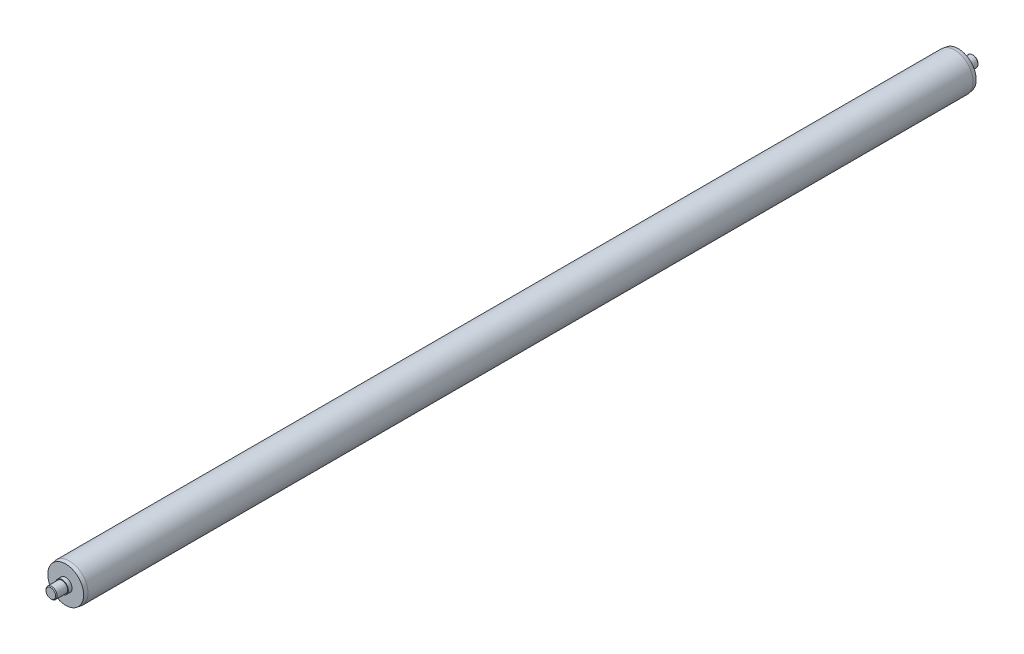
from build123d import *

# Parameters (mm, degrees)
CHAMFER1_SIZE  = 5
CHAMFER1_SIZE2 = 0.881634904
CHAMFER2_SIZE  = 1
SKETCH5_W      = 15.5
SKETCH5_H      = 1184


with BuildPart() as part:
    # Sketch3 → Revolve1 (revolve)
    with BuildSketch(Plane(origin=(0, 0, 0), x_dir=(0, 0, -1), z_dir=(1, 0, 0)), mode=Mode.PRIVATE) as revolve1_sk:
        Polygon((-300, 25), (900, 25), (900, 8.5), (905, 8.5), (905, 7.5), (920, 7.5), (920, 0), (-320, 0), (-320, 7.5), (-305, 7.5), (-305, 8.5), (-300, 8.5), align=None)
    revolve(revolve1_sk.sketch.rotate(Axis((0, 0, 320), (0, 0, -1)), 90), axis=Axis((0, 0, 320), (0, 0, -1)))

    # Chamfer1
    chamfer1_edges = [part.edges().sort_by_distance(p)[0] for p in [
        (-25, 0, -900),
        (-25, 0, 300),
    ]]
    chamfer1_side = [part.faces().sort_by_distance(p)[0] for p in [
        (-25, 0, -300),
    ]]
    chamfer(chamfer1_edges, length=CHAMFER1_SIZE, length2=CHAMFER1_SIZE2, reference=chamfer1_side[0])

    # Chamfer2
    chamfer2_edges = [part.edges().sort_by_distance(p)[0] for p in [
        (-7.5, 0, -920),
        (-7.5, 0, 320),
    ]]
    chamfer(chamfer2_edges, length=CHAMFER2_SIZE)

    # Sketch5 → Cut-Revolve1 (revolve, cut)
    with BuildSketch(Plane(origin=(0, 0, 0), x_dir=(1, 0, 0), z_dir=(0, 1, 0)), mode=Mode.PRIVATE) as cut_revolve1_sk:
        with Locations((15.25, 300)):
            Rectangle(SKETCH5_W, SKETCH5_H)
    revolve(cut_revolve1_sk.sketch.rotate(Axis((0, 0, -920), (0, 0, 1)), 180), axis=Axis((0, 0, -920), (0, 0, 1)), mode=Mode.SUBTRACT)


solid = part.part
